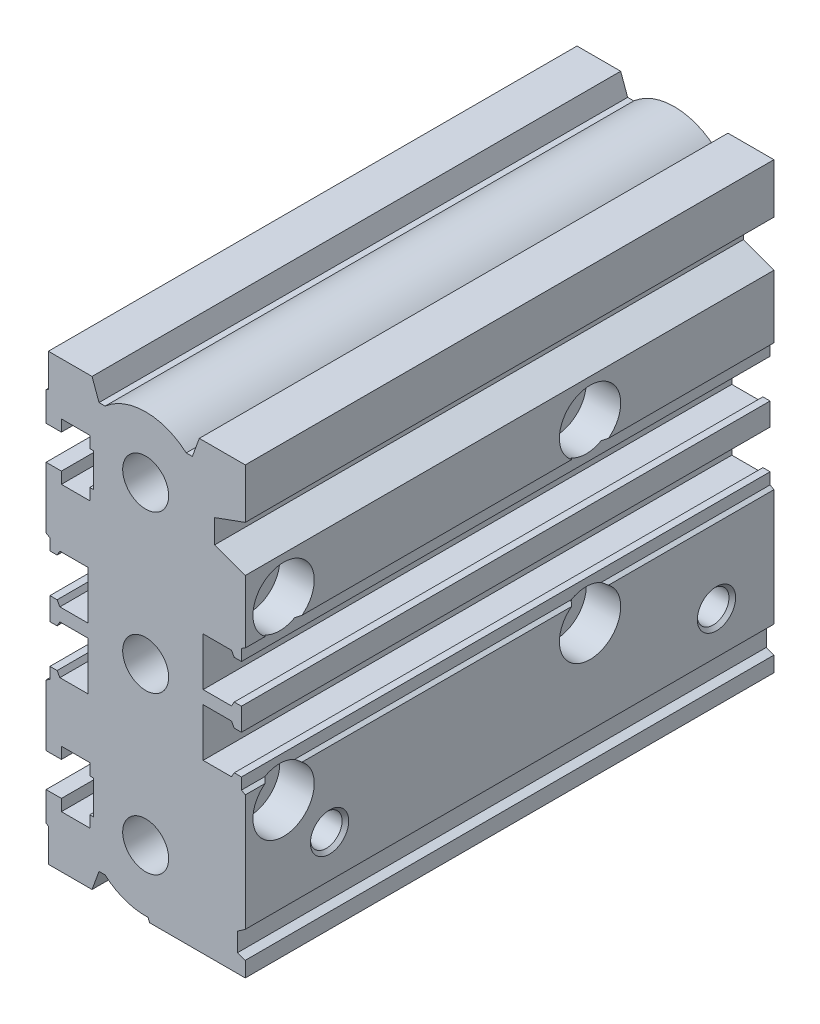
from build123d import *

# Parameters (mm, degrees)
SKETCH_1_W           = 26
SKETCH_1_H           = 58
EXTRUDE_1_DEPTH      = 69
SKETCH_2_R           = 3
CUT_EXTRUDE_1_DEPTH  = 69
SKETCH_3_R           = 3
CUT_EXTRUDE_2_DEPTH  = 69
SKETCH_4_R           = 3
CUT_EXTRUDE_3_DEPTH  = 14.5
SKETCH_5_R           = 6
CUT_EXTRUDE_4_DEPTH  = 45
CUT_EXTRUDE_5_DEPTH  = 3
CUT_EXTRUDE_6_DEPTH  = 3
CUT_EXTRUDE_7_DEPTH  = 69
CUT_EXTRUDE_8_DEPTH  = 69
SKETCH_26_W          = 28
SKETCH_26_H          = 60
CUT_EXTRUDE_9_DEPTH  = 69
SKETCH_27_W          = 28
SKETCH_27_H          = 60
CUT_EXTRUDE_10_DEPTH = 69


with BuildPart() as part:
    # 草图1 → 凸台-拉伸1 (new body)
    with BuildSketch(Plane.XY):
        Rectangle(SKETCH_1_W, SKETCH_1_H)
    extrude(amount=-EXTRUDE_1_DEPTH)

    # 草图2 → 切除-拉伸1 (cut)
    with BuildSketch(Plane.XY):
        with Locations((0, 20.5)):
            Circle(SKETCH_2_R)
    extrude(amount=-CUT_EXTRUDE_1_DEPTH, mode=Mode.SUBTRACT)

    # 草图3 → 切除-拉伸2 (cut)
    with BuildSketch(Plane.XY):
        with Locations((0, -20.5)):
            Circle(SKETCH_3_R)
    extrude(amount=-CUT_EXTRUDE_2_DEPTH, mode=Mode.SUBTRACT)

    # 草图4 → 切除-拉伸3 (cut)
    with BuildSketch(Plane.XY):
        Circle(SKETCH_4_R)
    extrude(amount=-CUT_EXTRUDE_3_DEPTH, mode=Mode.SUBTRACT)

    # 草图5 → 切除-拉伸4 (cut)
    with BuildSketch(Plane.XY.offset(-12)):
        Circle(SKETCH_5_R)
    extrude(amount=-CUT_EXTRUDE_4_DEPTH, mode=Mode.SUBTRACT)

    # 草图6 → 切除-旋转1 (revolve, cut)
    with BuildSketch(Plane(origin=(0, 11.5, 0), x_dir=(1, 0, 0), z_dir=(0, 1, 0)), mode=Mode.PRIVATE) as cut_revolve_1_sk:
        Polygon((-13, 5), (-13, 7.5), (-12.567, 7.067), (-3, 7.067), (-3, 7.15), (8.5, 7.15), (8.5, 9), (13, 9), (13, 5), align=None)
    revolve(cut_revolve_1_sk.sketch.rotate(Axis((13, 11.5, -5), (-1, 0, 0)), 180), axis=Axis((13, 11.5, -5), (-1, 0, 0)), mode=Mode.SUBTRACT)

    # 草图7 → 切除-旋转2 (revolve, cut)
    with BuildSketch(Plane(origin=(0, 11.5, 0), x_dir=(1, 0, 0), z_dir=(0, 1, 0)), mode=Mode.PRIVATE) as cut_revolve_2_sk:
        Polygon((-13, 45), (-13, 47.5), (-12.567, 47.067), (-3, 47.067), (-3, 47.15), (8.5, 47.15), (8.5, 49), (13, 49), (13, 45), align=None)
    revolve(cut_revolve_2_sk.sketch.rotate(Axis((13, 11.5, -45), (-1, 0, 0)), 180), axis=Axis((13, 11.5, -45), (-1, 0, 0)), mode=Mode.SUBTRACT)

    # 草图8 → 切除-旋转3 (revolve, cut)
    with BuildSketch(Plane(origin=(0, -11.5, 0), x_dir=(1, 0, 0), z_dir=(0, 1, 0)), mode=Mode.PRIVATE) as cut_revolve_3_sk:
        Polygon((-13, 45), (-13, 47.5), (-12.567, 47.067), (-3, 47.067), (-3, 47.15), (8.5, 47.15), (8.5, 49), (13, 49), (13, 45), align=None)
    revolve(cut_revolve_3_sk.sketch.rotate(Axis((13, -11.5, -45), (-1, 0, 0)), 180), axis=Axis((13, -11.5, -45), (-1, 0, 0)), mode=Mode.SUBTRACT)

    # 草图9 → 切除-旋转4 (revolve, cut)
    with BuildSketch(Plane(origin=(0, -11.5, 0), x_dir=(1, 0, 0), z_dir=(0, 1, 0)), mode=Mode.PRIVATE) as cut_revolve_4_sk:
        Polygon((-13, 5), (-13, 7.5), (-12.567, 7.067), (-3, 7.067), (-3, 7.15), (8.5, 7.15), (8.5, 9), (13, 9), (13, 5), align=None)
    revolve(cut_revolve_4_sk.sketch.rotate(Axis((13, -11.5, -5), (-1, 0, 0)), 180), axis=Axis((13, -11.5, -5), (-1, 0, 0)), mode=Mode.SUBTRACT)

    # 草图10 → 切除-旋转5 (revolve, cut)
    with BuildSketch(Plane(origin=(0, -18, 0), x_dir=(1, 0, 0), z_dir=(0, 1, 0)), mode=Mode.PRIVATE) as cut_revolve_5_sk:
        Polygon((3.806616994, 11), (5, 13.067), (12.567, 13.067), (13, 13.5), (13, 11), align=None)
    revolve(cut_revolve_5_sk.sketch.rotate(Axis((13, -18, -11), (-1, 0, 0)), 180), axis=Axis((13, -18, -11), (-1, 0, 0)), mode=Mode.SUBTRACT)

    # 草图11 → 切除-旋转6 (revolve, cut)
    with BuildSketch(Plane(origin=(0, -18, 0), x_dir=(1, 0, 0), z_dir=(0, 1, 0)), mode=Mode.PRIVATE) as cut_revolve_6_sk:
        Polygon((3.806616994, 61.5), (5, 63.567), (12.567, 63.567), (13, 64), (13, 61.5), align=None)
    revolve(cut_revolve_6_sk.sketch.rotate(Axis((13, -18, -61.5), (-1, 0, 0)), 180), axis=Axis((13, -18, -61.5), (-1, 0, 0)), mode=Mode.SUBTRACT)

    # 草图12 → 切除-旋转7 (revolve, cut)
    with BuildSketch(Plane(origin=(8, 0, 0), x_dir=(0, 0, -1), z_dir=(1, 0, 0)), mode=Mode.PRIVATE) as cut_revolve_7_sk:
        Polygon((11, -19.806616994), (13.067, -21), (13.067, -28.567), (13.5, -29), (11, -29), align=None)
    revolve(cut_revolve_7_sk.sketch.rotate(Axis((8, -29, -11), (0, 1, 0)), 180), axis=Axis((8, -29, -11), (0, 1, 0)), mode=Mode.SUBTRACT)

    # 草图13 → 切除-旋转8 (revolve, cut)
    with BuildSketch(Plane(origin=(8, 0, 0), x_dir=(0, 0, -1), z_dir=(1, 0, 0)), mode=Mode.PRIVATE) as cut_revolve_8_sk:
        Polygon((53, -19.806616994), (55.067, -21), (55.067, -28.567), (55.5, -29), (53, -29), align=None)
    revolve(cut_revolve_8_sk.sketch.rotate(Axis((8, -29, -53), (0, 1, 0)), 180), axis=Axis((8, -29, -53), (0, 1, 0)), mode=Mode.SUBTRACT)

    # 草图14 → 切除-旋转9 (revolve, cut)
    with BuildSketch(Plane.XY.offset(-25), mode=Mode.PRIVATE) as cut_revolve_9_sk:
        Polygon((-13, -11.5), (-13, -10), (-7, -10), (-6.133974596, -11.5), align=None)
    revolve(cut_revolve_9_sk.sketch.rotate(Axis((-6.133974596, -11.5, -25), (-1, 0, 0)), 270), axis=Axis((-6.133974596, -11.5, -25), (-1, 0, 0)), mode=Mode.SUBTRACT)

    # 草图15 → 切除-旋转10 (revolve, cut)
    with BuildSketch(Plane.XY.offset(-25), mode=Mode.PRIVATE) as cut_revolve_10_sk:
        Polygon((-13, 11.5), (-13, 13), (-7, 13), (-6.133974596, 11.5), align=None)
    revolve(cut_revolve_10_sk.sketch.rotate(Axis((-6.133974596, 11.5, -25), (-1, 0, 0)), 270), axis=Axis((-6.133974596, 11.5, -25), (-1, 0, 0)), mode=Mode.SUBTRACT)

    # 草图16 → 切除-拉伸5 (cut)
    with BuildSketch(Plane(origin=(-13, 0, 0), x_dir=(0, 0, -1), z_dir=(1, 0, 0))):
        with BuildLine():
            Line((26.5, 11.25), (26.5, 11.75))
            ThreePointArc((26.5, 11.75), (25, 13.25), (23.5, 11.75))
            Line((23.5, 11.75), (23.5, 11.25))
            ThreePointArc((23.5, 11.25), (25, 9.75), (26.5, 11.25))
        make_face()
    extrude(amount=CUT_EXTRUDE_5_DEPTH, mode=Mode.SUBTRACT)

    # 草图17 → 切除-旋转11 (revolve, cut)
    with BuildSketch(Plane(origin=(0, 25, 0), x_dir=(1, 0, 0), z_dir=(0, 1, 0)), mode=Mode.PRIVATE) as cut_revolve_11_sk:
        Polygon((9, 59), (7.379, 59), (7.379, 68.621), (7, 69), (9, 69), align=None)
    revolve(cut_revolve_11_sk.sketch.rotate(Axis((9, 25, -69), (0, 0, 1)), 180), axis=Axis((9, 25, -69), (0, 0, 1)), mode=Mode.SUBTRACT)

    # 草图18 → 切除-旋转12 (revolve, cut)
    with BuildSketch(Plane(origin=(0, -25, 0), x_dir=(1, 0, 0), z_dir=(0, 1, 0)), mode=Mode.PRIVATE) as cut_revolve_12_sk:
        Polygon((-9, 59), (-10.621, 59), (-10.621, 68.621), (-11, 69), (-9, 69), align=None)
    revolve(cut_revolve_12_sk.sketch.rotate(Axis((-9, -25, -69), (0, 0, 1)), 180), axis=Axis((-9, -25, -69), (0, 0, 1)), mode=Mode.SUBTRACT)

    # 草图19 → 切除-旋转13 (revolve, cut)
    with BuildSketch(Plane(origin=(0, -25, 0), x_dir=(1, 0, 0), z_dir=(0, 1, 0)), mode=Mode.PRIVATE) as cut_revolve_13_sk:
        Polygon((9, 59), (7.379, 59), (7.379, 68.621), (7, 69), (9, 69), align=None)
    revolve(cut_revolve_13_sk.sketch.rotate(Axis((9, -25, -69), (0, 0, 1)), 180), axis=Axis((9, -25, -69), (0, 0, 1)), mode=Mode.SUBTRACT)

    # 草图20 → 切除-旋转14 (revolve, cut)
    with BuildSketch(Plane(origin=(0, 25, 0), x_dir=(1, 0, 0), z_dir=(0, 1, 0)), mode=Mode.PRIVATE) as cut_revolve_14_sk:
        Polygon((-9, 59), (-10.621, 59), (-10.621, 68.621), (-11, 69), (-9, 69), align=None)
    revolve(cut_revolve_14_sk.sketch.rotate(Axis((-9, 25, -69), (0, 0, 1)), 180), axis=Axis((-9, 25, -69), (0, 0, 1)), mode=Mode.SUBTRACT)

    # 草图21 → 切除-旋转15 (revolve, cut)
    with BuildSketch(Plane(origin=(0, 0, 0), x_dir=(0, 0, -1), z_dir=(1, 0, 0)), mode=Mode.PRIVATE) as cut_revolve_15_sk:
        Polygon((62.133974596, -11.5), (63, -10), (69, -10), (69, -11.5), align=None)
    revolve(cut_revolve_15_sk.sketch.rotate(Axis((0, -11.5, -69), (0, 0, 1)), 270), axis=Axis((0, -11.5, -69), (0, 0, 1)), mode=Mode.SUBTRACT)

    # 草图22 → 切除-旋转16 (revolve, cut)
    with BuildSketch(Plane(origin=(0, 0, 0), x_dir=(0, 0, -1), z_dir=(1, 0, 0)), mode=Mode.PRIVATE) as cut_revolve_16_sk:
        Polygon((62.133974596, 11.5), (63, 13), (69, 13), (69, 11.5), align=None)
    revolve(cut_revolve_16_sk.sketch.rotate(Axis((0, 11.5, -69), (0, 0, 1)), 270), axis=Axis((0, 11.5, -69), (0, 0, 1)), mode=Mode.SUBTRACT)

    # 草图23 → 切除-拉伸6 (cut)
    with BuildSketch(Plane.XY.offset(-69)):
        with BuildLine():
            Line((1.5, 11.25), (1.5, 11.75))
            ThreePointArc((1.5, 11.75), (0, 13.25), (-1.5, 11.75))
            Line((-1.5, 11.75), (-1.5, 11.25))
            ThreePointArc((-1.5, 11.25), (0, 9.75), (1.5, 11.25))
        make_face()
    extrude(amount=CUT_EXTRUDE_6_DEPTH, mode=Mode.SUBTRACT)

    # 草图24 → 切除-拉伸7 (cut)
    with BuildSketch(Plane.XY.offset(-69)):
        Polygon((-13, 16.3), (-11, 16.3), (-11, 14.8), (-7.3, 14.8), (-7.3, 16.3), (-6.8, 16.3), (-6.8, 20.7), (-7.3, 20.7), (-7.3, 22.2), (-11, 22.2), (-11, 20.7), (-13, 20.7), align=None)
    extrude(amount=CUT_EXTRUDE_7_DEPTH, mode=Mode.SUBTRACT)

    # 草图25 → 切除-拉伸8 (cut)
    with BuildSketch(Plane.XY.offset(-69)):
        Polygon((-13, -20.7), (-11, -20.7), (-11, -22.2), (-7.3, -22.2), (-7.3, -20.7), (-6.8, -20.7), (-6.8, -16.3), (-7.3, -16.3), (-7.3, -14.8), (-11, -14.8), (-11, -16.3), (-13, -16.3), align=None)
    extrude(amount=CUT_EXTRUDE_8_DEPTH, mode=Mode.SUBTRACT)

    # 草图26 → 切除-拉伸9 (cut)
    with BuildSketch(Plane.XY.offset(-69)):
        Rectangle(SKETCH_26_W, SKETCH_26_H)
        with BuildLine():
            Line((-13, -24.5), (-12.7, -24.673205081))
            Line((-12.7, -24.673205081), (-12.7, -29))
            Line((-12.7, -29), (-7, -29))
            Line((-7, -29), (-6.090074414, -26.5))
            Line((-6.090074414, -26.5), (-5.291502622, -26.5))
            ThreePointArc((-5.291502622, -26.5), (-2.680170616, -28.037684357), (0.315746109, -28.493766596))
            Line((0.315746109, -28.493766596), (0.5, -29))
            Line((0.5, -29), (13, -29))
            Line((13, -29), (13, -27))
            Line((13, -27), (12, -26.636029766))
            Line((12, -26.636029766), (12, -24.200207538))
            Line((12, -24.200207538), (13, -23.5))
            Line((13, -23.5), (13, -8.3))
            Line((13, -8.3), (12.5, -8.011324865))
            Line((12.5, -8.011324865), (12.5, 8.011324865))
            Line((12.5, 8.011324865), (13, 8.3))
            Line((13, 8.3), (13, 16.5))
            Line((13, 16.5), (9, 17.955880937))
            Line((9, 17.955880937), (9, 21.044119063))
            Line((9, 21.044119063), (13, 22.5))
            Line((13, 22.5), (13, 29))
            Line((13, 29), (7, 29))
            Line((7, 29), (6.090074414, 26.5))
            Line((6.090074414, 26.5), (5.291502622, 26.5))
            ThreePointArc((5.291502622, 26.5), (0, 28.5), (-5.291502622, 26.5))
            Line((-5.291502622, 26.5), (-6.090074414, 26.5))
            Line((-6.090074414, 26.5), (-7, 29))
            Line((-7, 29), (-12.7, 29))
            Line((-12.7, 29), (-12.7, 24.673205081))
            Line((-12.7, 24.673205081), (-13, 24.5))
            Line((-13, 24.5), (-13, 8.3))
            Line((-13, 8.3), (-12.5, 8.011324865))
            Line((-12.5, 8.011324865), (-12.5, -8.011324865))
            Line((-12.5, -8.011324865), (-13, -8.3))
            Line((-13, -8.3), (-13, -24.5))
        make_face(mode=Mode.SUBTRACT)
    extrude(amount=CUT_EXTRUDE_9_DEPTH, mode=Mode.SUBTRACT)

    # 草图27 → 切除-拉伸10 (cut)
    with BuildSketch(Plane.XY):
        Rectangle(SKETCH_27_W, SKETCH_27_H)
        Polygon((-13, 6.525), (-11.560843918, 6.525), (-11.2, 7.15), (-7.5, 7.15), (-7.5, 0.85), (-11.2, 0.85), (-11.560843918, 1.475), (-13, 1.475), (-13, -1.475), (-11.560843918, -1.475), (-11.2, -0.85), (-7.5, -0.85), (-7.5, -7.15), (-11.2, -7.15), (-11.560843918, -6.525), (-13, -6.525), (-13, -29), (13, -29), (13, -6.525), (11.560843918, -6.525), (11.2, -7.15), (7.5, -7.15), (7.5, -0.85), (11.2, -0.85), (11.560843918, -1.475), (13, -1.475), (13, 1.475), (11.560843918, 1.475), (11.2, 0.85), (7.5, 0.85), (7.5, 7.15), (11.2, 7.15), (11.560843918, 6.525), (13, 6.525), (13, 29), (-13, 29), align=None, mode=Mode.SUBTRACT)
    extrude(amount=-CUT_EXTRUDE_10_DEPTH, mode=Mode.SUBTRACT)


solid = part.part
